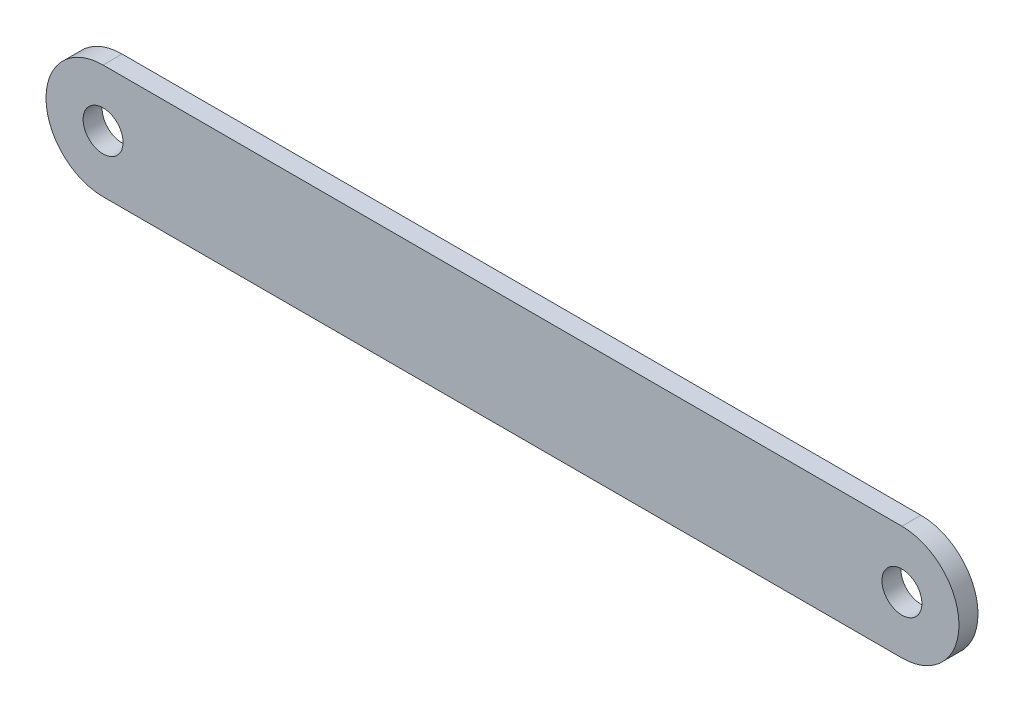
from build123d import *

# Parameters (mm, degrees)
BOSS_EXTRUDE1_DEPTH        = 1
F_4_2_4_2_DIAMETER_HOLE1_D = 4.2


with BuildPart() as part:
    # Sketch1 → Boss-Extrude1 (new, symmetric)
    with BuildSketch(Plane.XY):
        with BuildLine():
            Line((0, 6), (84, 6))
            ThreePointArc((84, 6), (90, 0), (84, -6))
            Line((84, -6), (0, -6))
            ThreePointArc((0, -6), (-6, 0), (0, 6))
        make_face()
    extrude(amount=BOSS_EXTRUDE1_DEPTH, both=True)

    # Ø4.2 (4.2) Diameter Hole1 (through all)
    with Locations(Plane.XY.offset(1)):
        with Locations((0, 0), (84, 0)):
            Hole(F_4_2_4_2_DIAMETER_HOLE1_D / 2)


solid = part.part
